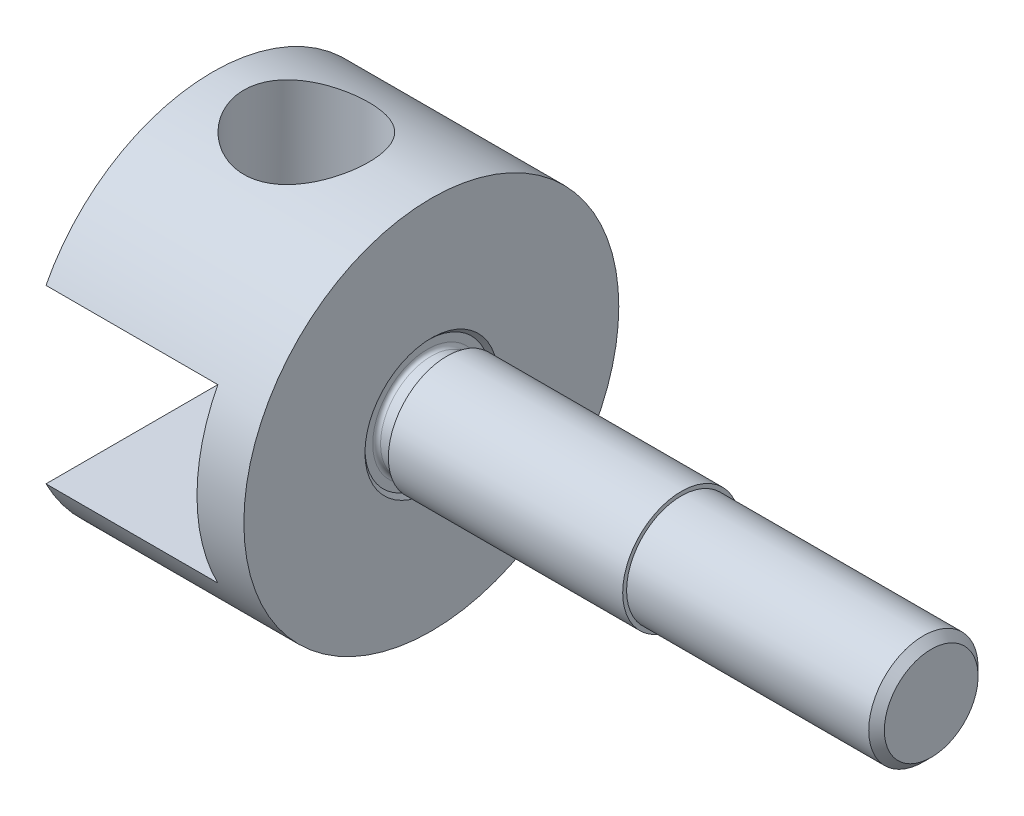
from build123d import *

# Parameters (mm, degrees)
SKETCH2_W               = 84.798069866
SKETCH2_H               = 22
CUT_EXTRUDE1_DEPTH      = 22
CUT_EXTRUDE2_DEPTH      = 51
CUT_EXTRUDE2_DEPTH_BACK = 22
SKETCH3_R               = 8
CHAMFER1_SIZE           = 1


with BuildPart() as part:
    # Sketch1 → Revolve1 (revolve)
    with BuildSketch(Plane.XY, mode=Mode.PRIVATE) as revolve1_sk:
        Polygon((0, 0), (0, 24), (28, 24), (28, 7), (30, 7), (30, 7.5), (60, 7.5), (60, 7), (92, 7), (92, 0), align=None)
    revolve(revolve1_sk.sketch.rotate(Axis((-36.181818182, 0, 0), (1, 0, 0)), 90), axis=Axis((-36.181818182, 0, 0), (1, 0, 0)))

    # Sketch2 → Cut-Extrude1 (cut)
    with BuildSketch(Plane.ZY):
        Rectangle(SKETCH2_W, SKETCH2_H)
    extrude(amount=-CUT_EXTRUDE1_DEPTH, mode=Mode.SUBTRACT)

    # Sketch3 → Cut-Extrude2 (cut, two sides: drawn at the far end of the back side and taken through both)
    with BuildSketch(Plane(origin=(0, -11, 0), x_dir=(1, 0, 0), z_dir=(0, 1, 0)).offset(-CUT_EXTRUDE2_DEPTH_BACK)):
        with Locations(Location((12, 0, 0), (0, 0, 90))):
            Circle(SKETCH3_R)
    extrude(amount=CUT_EXTRUDE2_DEPTH + CUT_EXTRUDE2_DEPTH_BACK, mode=Mode.SUBTRACT)

    # Sketch7 → Cut-Revolve1 (revolve, cut)
    with BuildSketch(Plane(origin=(0, 0, 0), x_dir=(1, 0, 0), z_dir=(0, 1, 0))):
        with BuildLine():
            Line((28, -6.5), (29.5, -6.5))
            Line((29.5, -6.5), (30, -7))
            Line((30, -7), (28, -7))
            Line((28, -7), (28, -8.5))
            Line((28, -8.5), (27.5, -8))
            Line((27.5, -8), (27.5, -7))
            ThreePointArc((27.5, -7), (27.646446609, -6.646446609), (28, -6.5))
        make_face()
    revolve(axis=Axis((0, 0, 0), (1, 0, 0)), mode=Mode.SUBTRACT)

    # Chamfer1
    chamfer1_edges = [part.edges().sort_by_distance(p)[0] for p in [
        (92, 0, -7),
    ]]
    chamfer(chamfer1_edges, length=CHAMFER1_SIZE)


solid = part.part
